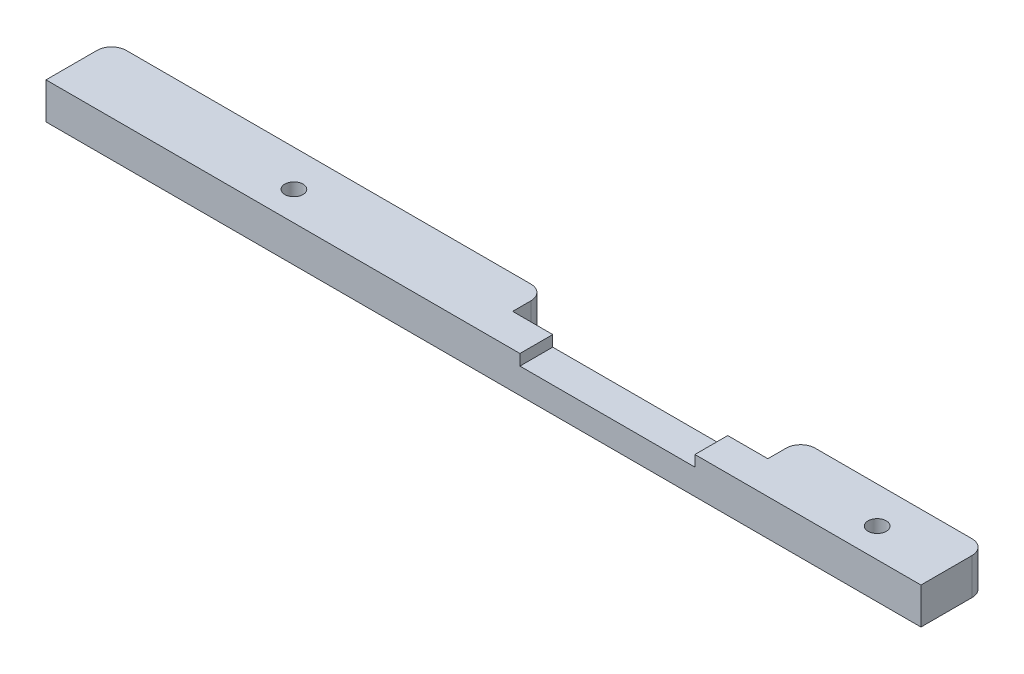
from build123d import *

# Parameters (mm, degrees)
SKETCH1_W             = 120
SKETCH1_H             = 9
BOSS_EXTRUDE1_DEPTH   = 5
M3_TAPPED_HOLE1_D     = 2.5
M3_TAPPED_HOLE1_DEPTH = 8.5
FILLET1_R             = 2
SKETCH4_W             = 35
SKETCH4_H             = 4.5
CUT_EXTRUDE1_DEPTH    = 121.440856855
FILLET2_R             = 2
SKETCH5_W             = 24
SKETCH5_H             = 9
CUT_EXTRUDE2_DEPTH    = 1.5


with BuildPart() as part:
    # Sketch1 → Boss-Extrude1 (new body)
    with BuildSketch(Plane(origin=(0, 0, 0), x_dir=(1, 0, 0), z_dir=(0, 1, 0))):
        with Locations((60, 4.5)):
            Rectangle(SKETCH1_W, SKETCH1_H)
    extrude(amount=BOSS_EXTRUDE1_DEPTH)

    # M3 Tapped Hole1
    with Locations(Plane(origin=(0, 5, 0), x_dir=(-1, 0, 0), z_dir=(0, 1, 0))):
        with Locations((-30, -4), (-110, -4)):
            Hole(M3_TAPPED_HOLE1_D / 2, depth=M3_TAPPED_HOLE1_DEPTH)

    # Fillet1
    fillet1_edges = [part.edges().sort_by_distance(p)[0] for p in [
        (0, 2.5, -9),
        (120, 2.5, -9),
    ]]
    fillet(fillet1_edges, radius=FILLET1_R)

    # Sketch4 → Cut-Extrude1 (cut, through all)
    with BuildSketch(Plane(origin=(0, 5, 0), x_dir=(-1, 0, 0), z_dir=(0, 1, 0))):
        with Locations((-77, -6.75)):
            Rectangle(SKETCH4_W, SKETCH4_H)
    extrude(amount=-CUT_EXTRUDE1_DEPTH, mode=Mode.SUBTRACT)

    # Fillet2
    fillet2_edges = [part.edges().sort_by_distance(p)[0] for p in [
        (94.5, 2.5, -9),
        (59.5, 2.5, -9),
    ]]
    fillet(fillet2_edges, radius=FILLET2_R)

    # Sketch5 → Cut-Extrude2 (cut)
    with BuildSketch(Plane.XZ.offset(-5)):
        with Locations((77, -4.5)):
            Rectangle(SKETCH5_W, SKETCH5_H)
    extrude(amount=CUT_EXTRUDE2_DEPTH, mode=Mode.SUBTRACT)


solid = part.part
